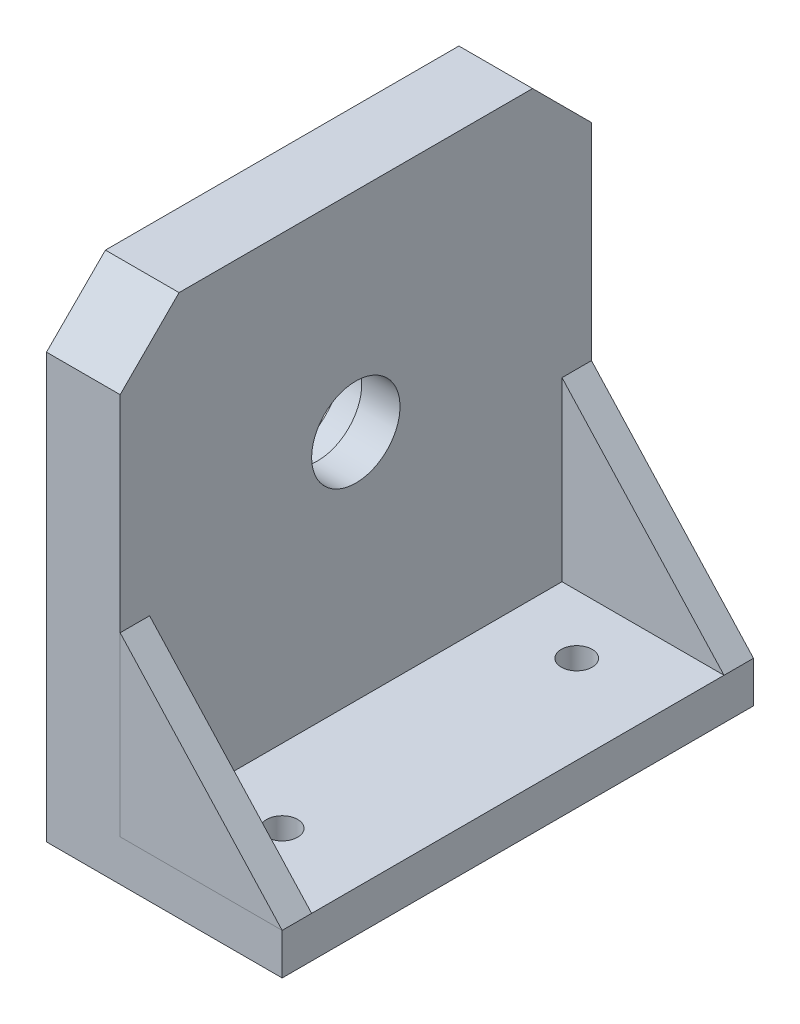
SolidWorks part; units mm, degrees
ref_plane "前视基准面" through (0, 0, 0) normal (0, 0, 1) x (1, 0, 0)
ref_plane "上视基准面" through (0, 0, 0) normal (0, 1, 0) x (1, 0, 0)
ref_plane "右视基准面" through (0, 0, 0) normal (1, 0, 0) x (0, 0, -1)
sketch "草图1" plane through (0, 0, 0) normal (0, 1, 0) x (1, 0, 0)
  line L1 (-40, 80) -> (40, 80)
  line L2 (-40, 80) -> (-40, -80)
  line L3 (-40, -80) -> (40, -80)
  line L4 (40, 80) -> (40, -80)
  line L5 (-40, 80) -> (40, -80) construction
  line L6 (-40, -80) -> (40, 80) construction
  point P0 (0, 0)
  dimension "D1" = 80
  dimension "D2" = 160
extrude "凸台-拉伸1" add sketch "草图1" along normal blind 14
sketch "草图2" plane through (0, 14, 0) normal (0, 1, 0) x (1, 0, 0)
  line L0 (-40, -80) -> (40, -80) construction
  line L1 (-40, 80) -> (-15, 80)
  line L2 (-40, 80) -> (-40, -80)
  line L3 (-40, -80) -> (-15, -80)
  line L4 (-15, 80) -> (-15, -80)
  dimension "D1" = 25
extrude "凸台-拉伸2" add sketch "草图2" along normal blind 150
sketch "草图3" plane through (0, 0, 80) normal (0, 0, 1) x (1, 0, 0)
  line L0 (-15, 74) -> (40, 14)
  line L1 (-15, 164) -> (-15, 14) construction
  line L2 (-15, 14) -> (40, 14) construction
  line L3 (-15, 74) -> (-15, 14)
  line L4 (-15, 14) -> (40, 14)
  dimension "D1" = 60
extrude "凸台-拉伸3" add sketch "草图3" against normal blind 10 separate body
sketch "草图4" plane through (0, 0, -80) normal (0, 0, -1) x (-1, 0, 0)
  line L3 (15, 14) -> (15, 74)
  line L4 (15, 74) -> (-40, 14)
  line L5 (15, 14) -> (15, 74)
  line L7 (15, 74) -> (-40, 14)
  line L9 (-40, 14) -> (15, 14)
  line L10 (-40, 14) -> (15, 14)
  dimension "D1" = 0
extrude "凸台-拉伸4" add sketch "草图4" against normal blind 10 separate body
sketch "草图5" plane through (-40, 0, 0) normal (-1, 0, 0) x (0, 0, 1)
  line L0 (-80, 0) -> (80, 0) construction
  circle A0 centre (0, 93) radius 21
  dimension "D1" = 93
  dimension "D2" = 42
extrude "切除-拉伸1" cut sketch "草图5" against normal blind 12
sketch "草图6" plane through (-28, 0, 0) normal (-1, 0, 0) x (0, 0, 1)
  circle A0 centre (0, 93) radius 15
  dimension "D1" = 30
extrude "切除-拉伸2" cut sketch "草图6" against normal through all
hole_wizard "Ø10.5 (10.5) 直径孔1" positions "草图8" profile "草图9" hole size "Ø10.5" standard "GB"
sketch "草图8" plane through (0, 14, 0) normal (0, 1, 0) x (1, 0, 0)
  line L0 (0, 0) -> (45.5582, 0) construction
  line L2 (40, -80) -> (40, 80) construction
  point P0 (10, 50)
  point P2 (10, -50)
  dimension "D1" = 100
  dimension "D2" = 30
sketch "草图9" plane through (10, 14, -50) normal (1, 0, 0) x (0, 0, 1)
  line L0 (0, 0) -> (0, 18.1545)
  line L1 (0, 18.1545) -> (5.25, 15)
  line L2 (5.25, 15) -> (5.25, 0)
  line L5 (5.25, 0) -> (0, 0)
  line L10 (0, 18.1545) -> (-5.25, 15) construction
  line L11 (0, -6.35) -> (0, 107.95) construction
  dimension "孔直径" = 10.5
  dimension "孔深度" = 15
  dimension "导头角度" = 118
chamfer "倒角1" distance 20 angle 45 2 edges at (-27.5, 164, 80) (-27.5, 164, -80)
